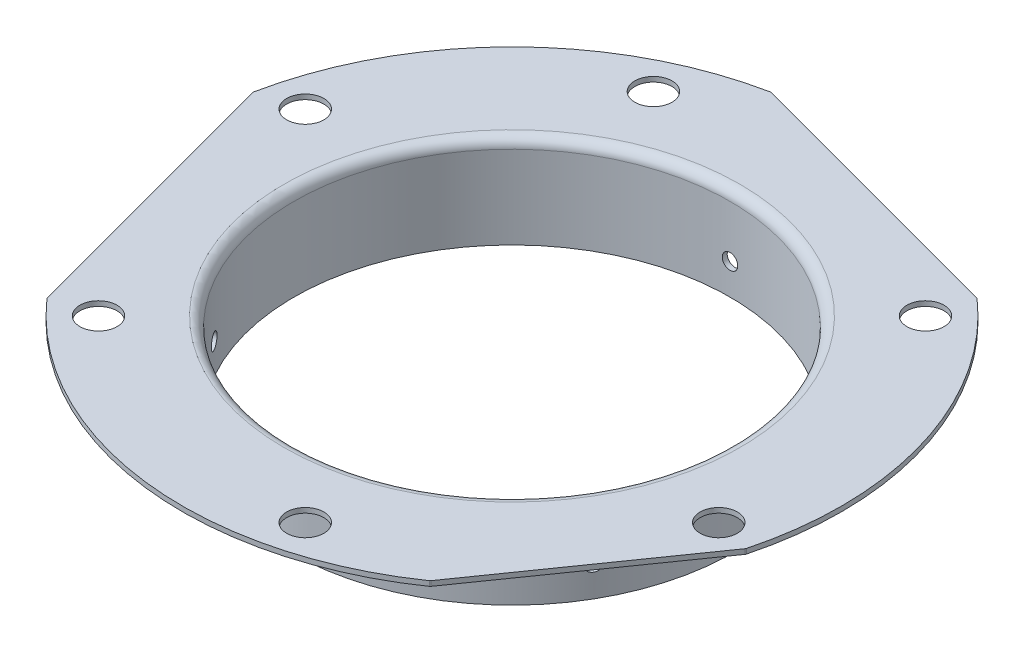
from build123d import *

# Parameters (mm, degrees)
CUT_EXTRUDE1_REACH      = 155.572
SKETCH2_R               = 6
CUT_EXTRUDE2_REACH      = 155.572
FILLET1_R               = 1
CUT_EXTRUDE3_REACH      = 155.572
CUT_EXTRUDE3_END_RADIUS = 72.1
SKETCH4_R               = 2.5
CIRPATTERN1_COUNT       = 3


with BuildPart() as part:
    # Sketch1 → Revolve1 (revolve)
    with BuildSketch(Plane(origin=(0, 0, 0), x_dir=(0, 0, -1), z_dir=(1, 0, 0))):
        with BuildLine():
            Line((-106.5, 0), (-73.7, 0))
            ThreePointArc((-73.7, 0), (-71.4372583, -0.9372583), (-70.5, -3.2))
            Line((-70.5, -3.2), (-70.5, -30))
            Line((-70.5, -30), (-72.1, -30))
            Line((-72.1, -30), (-72.1, -3.2))
            ThreePointArc((-72.1, -3.2), (-72.56862915, -2.06862915), (-73.7, -1.6))
            Line((-73.7, -1.6), (-106.5, -1.6))
            Line((-106.5, -1.6), (-106.5, 0))
        make_face()
    revolve(axis=Axis((0, 0, 0), (0, -1, 0)))

    # Sketch2 → Cut-Extrude1 (cut, up to next)
    with BuildSketch(Plane(origin=(0, 0, 0), x_dir=(1, 0, 0), z_dir=(0, 1, 0)), mode=Mode.PRIVATE) as cut_extrude1_sk1:
        with Locations(Location((-91.279990584, 24.458399762, 0), (0, 0, 270))):
            Circle(SKETCH2_R)
    cut_extrude1_tool1 = extrude(cut_extrude1_sk1.sketch, amount=-CUT_EXTRUDE1_REACH, mode=Mode.PRIVATE) & part.part
    # Sketch2 → Cut-Extrude1 (cut, up to next)
    with BuildSketch(Plane(origin=(0, 0, 0), x_dir=(1, 0, 0), z_dir=(0, 1, 0)), mode=Mode.PRIVATE) as cut_extrude1_sk2:
        with Locations(Location((-39.937425734, 85.646085875, 0), (0, 0, 270))):
            Circle(SKETCH2_R)
    cut_extrude1_tool2 = extrude(cut_extrude1_sk2.sketch, amount=-CUT_EXTRUDE1_REACH, mode=Mode.PRIVATE) & part.part
    # Sketch2 → Cut-Extrude1 (cut, up to next)
    with BuildSketch(Plane(origin=(0, 0, 0), x_dir=(1, 0, 0), z_dir=(0, 1, 0)), mode=Mode.PRIVATE) as cut_extrude1_sk3:
        with Locations(Location((66.821590822, 66.821590822, 0), (0, 0, 270))):
            Circle(SKETCH2_R)
    cut_extrude1_tool3 = extrude(cut_extrude1_sk3.sketch, amount=-CUT_EXTRUDE1_REACH, mode=Mode.PRIVATE) & part.part
    # Sketch2 → Cut-Extrude1 (cut, up to next)
    with BuildSketch(Plane(origin=(0, 0, 0), x_dir=(1, 0, 0), z_dir=(0, 1, 0)), mode=Mode.PRIVATE) as cut_extrude1_sk4:
        with Locations(Location((91.279990584, -24.458399762, 0), (0, 0, 270))):
            Circle(SKETCH2_R)
    cut_extrude1_tool4 = extrude(cut_extrude1_sk4.sketch, amount=-CUT_EXTRUDE1_REACH, mode=Mode.PRIVATE) & part.part
    # Sketch2 → Cut-Extrude1 (cut, up to next)
    with BuildSketch(Plane(origin=(0, 0, 0), x_dir=(1, 0, 0), z_dir=(0, 1, 0)), mode=Mode.PRIVATE) as cut_extrude1_sk5:
        with Locations(Location((24.458399762, -91.279990584, 0), (0, 0, 270))):
            Circle(SKETCH2_R)
    cut_extrude1_tool5 = extrude(cut_extrude1_sk5.sketch, amount=-CUT_EXTRUDE1_REACH, mode=Mode.PRIVATE) & part.part
    # Sketch2 → Cut-Extrude1 (cut, up to next)
    with BuildSketch(Plane(origin=(0, 0, 0), x_dir=(1, 0, 0), z_dir=(0, 1, 0)), mode=Mode.PRIVATE) as cut_extrude1_sk6:
        with Locations(Location((-66.821590822, -66.821590822, 0), (0, 0, 270))):
            Circle(SKETCH2_R)
    cut_extrude1_tool6 = extrude(cut_extrude1_sk6.sketch, amount=-CUT_EXTRUDE1_REACH, mode=Mode.PRIVATE) & part.part
    add(cut_extrude1_tool1.solids().sort_by_distance((-91.279991, 0, -24.4584))[0], mode=Mode.SUBTRACT)
    add(cut_extrude1_tool2.solids().sort_by_distance((-39.937426, 0, -85.646086))[0], mode=Mode.SUBTRACT)
    add(cut_extrude1_tool3.solids().sort_by_distance((66.821591, 0, -66.821591))[0], mode=Mode.SUBTRACT)
    add(cut_extrude1_tool4.solids().sort_by_distance((91.279991, 0, 24.4584))[0], mode=Mode.SUBTRACT)
    add(cut_extrude1_tool5.solids().sort_by_distance((24.4584, 0, 91.279991))[0], mode=Mode.SUBTRACT)
    add(cut_extrude1_tool6.solids().sort_by_distance((-66.821591, 0, 66.821591))[0], mode=Mode.SUBTRACT)

    # Sketch3 → Cut-Extrude2 (cut, up to next)
    with BuildSketch(Plane(origin=(0, 0, 0), x_dir=(1, 0, 0), z_dir=(0, 1, 0)), mode=Mode.PRIVATE) as cut_extrude2_sk1:
        with BuildLine():
            Line((-80.045679675, -70.249122168), (-104.446153146, 20.814684553))
            ThreePointArc((-104.446153146, 20.814684553), (-102.8711005, -27.564228303), (-80.045679675, -70.249122168))
        make_face()
    cut_extrude2_tool1 = extrude(cut_extrude2_sk1.sketch, amount=-CUT_EXTRUDE2_REACH, mode=Mode.PRIVATE) & part.part
    # Sketch3 → Cut-Extrude2 (cut, up to next)
    with BuildSketch(Plane(origin=(0, 0, 0), x_dir=(1, 0, 0), z_dir=(0, 1, 0)), mode=Mode.PRIVATE) as cut_extrude2_sk2:
        with BuildLine():
            Line((-20.814684553, 104.446153146), (70.249122168, 80.045679675))
            ThreePointArc((70.249122168, 80.045679675), (27.564228303, 102.8711005), (-20.814684553, 104.446153146))
        make_face()
    cut_extrude2_tool2 = extrude(cut_extrude2_sk2.sketch, amount=-CUT_EXTRUDE2_REACH, mode=Mode.PRIVATE) & part.part
    # Sketch3 → Cut-Extrude2 (cut, up to next)
    with BuildSketch(Plane(origin=(0, 0, 0), x_dir=(1, 0, 0), z_dir=(0, 1, 0)), mode=Mode.PRIVATE) as cut_extrude2_sk3:
        with BuildLine():
            Line((60.901239279, -87.368696077), (102.929169579, -27.346591193))
            ThreePointArc((102.929169579, -27.346591193), (87.239692717, -61.085890471), (60.901239279, -87.368696077))
        make_face()
    cut_extrude2_tool3 = extrude(cut_extrude2_sk3.sketch, amount=-CUT_EXTRUDE2_REACH, mode=Mode.PRIVATE) & part.part
    add(cut_extrude2_tool1.solids().sort_by_distance((-96.515383, 0, 25.861219))[0], mode=Mode.SUBTRACT)
    add(cut_extrude2_tool2.solids().sort_by_distance((25.861219, 0, -96.515383))[0], mode=Mode.SUBTRACT)
    add(cut_extrude2_tool3.solids().sort_by_distance((84.050671, 0, 58.852913))[0], mode=Mode.SUBTRACT)

    # Fillet1
    fillet1_edges = [part.edges().sort_by_distance(p)[0] for p in [
        (-80.045679675, -0.8, 70.249122168),
        (-104.446153146, -0.8, -20.814684553),
        (-20.814684553, -0.8, -104.446153146),
        (70.249122168, -0.8, -80.045679675),
        (102.929169579, -0.8, 27.346591193),
        (60.901239279, -0.8, 87.368696077),
    ]]
    fillet(fillet1_edges, radius=FILLET1_R)

    # Cut-Extrude3: up to this cylinder (the profile starts inside it)
    cut_extrude3_end = Plane(origin=(0, -20, 0), z_dir=(0, 1, 0)) * Cylinder(CUT_EXTRUDE3_END_RADIUS, 456.344, mode=Mode.PRIVATE)
    # Sketch4 → Cut-Extrude3 (cut, up to the surface)
    with BuildSketch(Plane.XY, mode=Mode.PRIVATE) as cut_extrude3_sk1:
        with Locations((0, -20)):
            Circle(SKETCH4_R)
    cut_extrude3_tool1 = extrude(cut_extrude3_sk1.sketch, amount=-CUT_EXTRUDE3_REACH, mode=Mode.PRIVATE) & cut_extrude3_end
    cut_extrude3 = cut_extrude3_tool1.solids().sort_by_distance((0, -20, 0))[0]
    add(cut_extrude3, mode=Mode.SUBTRACT)

    # CirPattern1: Cut-Extrude3 ×3 about axis
    cirpattern1_axis = Axis((0, -30, 0), (0, 1, 0))
    for i in range(1, CIRPATTERN1_COUNT):
        add(cut_extrude3.rotate(cirpattern1_axis, i * 360 / CIRPATTERN1_COUNT), mode=Mode.SUBTRACT)


solid = part.part
